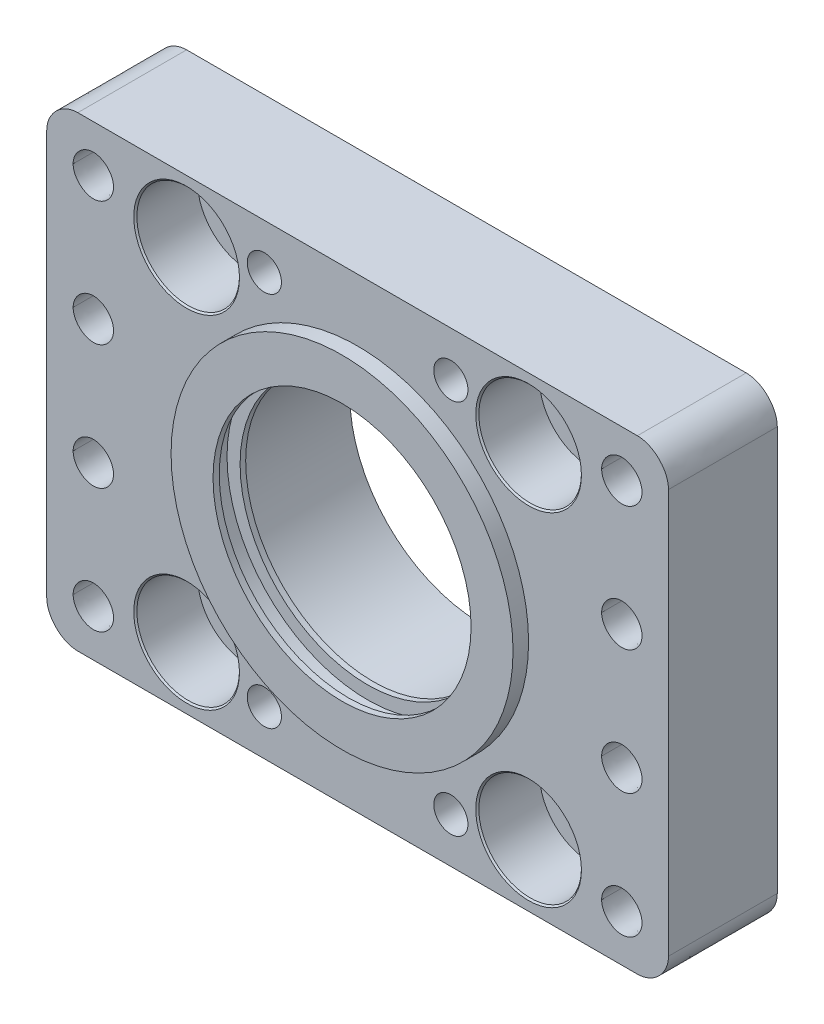
SolidWorks part; units mm, degrees
ref_plane "Front Plane" through (0, 0, 0) normal (0, 0, 1) x (1, 0, 0)
ref_plane "Top Plane" through (0, 0, 0) normal (0, 1, 0) x (1, 0, 0)
ref_plane "Right Plane" through (0, 0, 0) normal (1, 0, 0) x (0, 0, -1)
sketch "Sketch2" plane through (0, 0, 0) normal (0, 0, 1) x (1, 0, 0)
  circle A1 centre (48.7494, 55) radius 8.25
  spline S40 degree 3 poles (-53.0006, -55) (-53.0006, -59.3307) (-56.9229, -63.2494) (-65.5784, -63.2506) (-69.5006, -59.3366) (-69.5006, -55) knots 0 0 0 0 0.5 0.5 1 1 1 1
  spline S41 degree 3 poles (-69.5006, -55) (-69.5006, -50.6693) (-65.5784, -46.7506) (-56.9229, -46.7494) (-53.0006, -50.6634) (-53.0006, -55) knots 0 0 0 0 0.5 0.5 1 1 1 1
  spline S42 degree 3 poles (56.9994, -55) (56.9994, -59.3307) (53.0771, -63.2494) (44.4216, -63.2506) (40.4994, -59.3366) (40.4994, -55) knots 0 0 0 0 0.5 0.5 1 1 1 1
  spline S43 degree 3 poles (40.4994, -55) (40.4994, -50.6693) (44.4216, -46.7506) (53.0771, -46.7494) (56.9994, -50.6634) (56.9994, -55) knots 0 0 0 0 0.5 0.5 1 1 1 1
  spline S46 degree 3 poles (-53.0006, 55) (-53.0006, 50.6693) (-56.9229, 46.7506) (-65.5784, 46.7494) (-69.5006, 50.6634) (-69.5006, 55) knots 0 0 0 0 0.5 0.5 1 1 1 1
  spline S47 degree 3 poles (-69.5006, 55) (-69.5006, 59.3307) (-65.5784, 63.2494) (-56.9229, 63.2506) (-53.0006, 59.3366) (-53.0006, 55) knots 0 0 0 0 0.5 0.5 1 1 1 1
  spline S48 degree 3 poles (-84.7506, -60) (-84.7506, -63.4114) (-87.8428, -66.4994) (-94.6585, -66.5006) (-97.7506, -63.4173) (-97.7506, -60) knots 0 0 0 0 0.5 0.5 1 1 1 1
  spline S49 degree 3 poles (-97.7506, -60) (-97.7506, -56.5886) (-94.6585, -53.5006) (-87.8428, -53.4994) (-84.7506, -56.5827) (-84.7506, -60) knots 0 0 0 0 0.5 0.5 1 1 1 1
  spline S50 degree 3 poles (-84.7506, -20) (-84.7506, -23.4114) (-87.8428, -26.4994) (-94.6585, -26.5006) (-97.7506, -23.4173) (-97.7506, -20) knots 0 0 0 0 0.5 0.5 1 1 1 1
  spline S51 degree 3 poles (-97.7506, -20) (-97.7506, -16.5886) (-94.6585, -13.5006) (-87.8428, -13.4994) (-84.7506, -16.5827) (-84.7506, -20) knots 0 0 0 0 0.5 0.5 1 1 1 1
  spline S52 degree 3 poles (-84.7506, 20) (-84.7506, 16.5886) (-87.8428, 13.5006) (-94.6585, 13.4994) (-97.7506, 16.5827) (-97.7506, 20) knots 0 0 0 0 0.5 0.5 1 1 1 1
  spline S53 degree 3 poles (-97.7506, 20) (-97.7506, 23.4114) (-94.6585, 26.4994) (-87.8428, 26.5006) (-84.7506, 23.4173) (-84.7506, 20) knots 0 0 0 0 0.5 0.5 1 1 1 1
  spline S54 degree 3 poles (-84.7506, 60) (-84.7506, 56.5886) (-87.8428, 53.5006) (-94.6585, 53.4994) (-97.7506, 56.5827) (-97.7506, 60) knots 0 0 0 0 0.5 0.5 1 1 1 1
  spline S55 degree 3 poles (-97.7506, 60) (-97.7506, 63.4114) (-94.6585, 66.4994) (-87.8428, 66.5006) (-84.7506, 63.4173) (-84.7506, 60) knots 0 0 0 0 0.5 0.5 1 1 1 1
  spline S56 degree 3 poles (85.2494, -60) (85.2494, -63.4114) (82.1572, -66.4994) (75.3415, -66.5006) (72.2494, -63.4173) (72.2494, -60) knots 0 0 0 0 0.5 0.5 1 1 1 1
  spline S57 degree 3 poles (72.2494, -60) (72.2494, -56.5886) (75.3415, -53.5006) (82.1572, -53.4994) (85.2494, -56.5827) (85.2494, -60) knots 0 0 0 0 0.5 0.5 1 1 1 1
  spline S58 degree 3 poles (85.2494, -20) (85.2494, -23.4114) (82.1572, -26.4994) (75.3415, -26.5006) (72.2494, -23.4173) (72.2494, -20) knots 0 0 0 0 0.5 0.5 1 1 1 1
  spline S59 degree 3 poles (72.2494, -20) (72.2494, -16.5886) (75.3415, -13.5006) (82.1572, -13.4994) (85.2494, -16.5827) (85.2494, -20) knots 0 0 0 0 0.5 0.5 1 1 1 1
  spline S60 degree 3 poles (85.2494, 20) (85.2494, 16.5886) (82.1572, 13.5006) (75.3415, 13.4994) (72.2494, 16.5827) (72.2494, 20) knots 0 0 0 0 0.5 0.5 1 1 1 1
  spline S61 degree 3 poles (72.2494, 20) (72.2494, 23.4114) (75.3415, 26.4994) (82.1572, 26.5006) (85.2494, 23.4173) (85.2494, 20) knots 0 0 0 0 0.5 0.5 1 1 1 1
  spline S62 degree 3 poles (85.2494, 60) (85.2494, 56.5886) (82.1572, 53.5006) (75.3415, 53.4994) (72.2494, 56.5827) (72.2494, 60) knots 0 0 0 0 0.5 0.5 1 1 1 1
  spline S63 degree 3 poles (72.2494, 60) (72.2494, 63.4114) (75.3415, 66.4994) (82.1572, 66.5006) (85.2494, 63.4173) (85.2494, 60) knots 0 0 0 0 0.5 0.5 1 1 1 1
  spline S72 degree 3 poles (-106.2506, -65) (-106.2506, -21.6667) (-106.2506, 21.6667) (-106.2506, 65) knots 0 0 0 0 1 1 1 1
  spline S73 degree 3 poles (-96.2506, -75) (-101.4866, -75) (-106.2506, -70.236) (-106.2506, -65) knots 0 0 0 0 1 1 1 1
  spline S74 degree 3 poles (-96.2506, -75) (-36.2506, -75) (23.7494, -75) (83.7494, -75) knots 0 0 0 0 1 1 1 1
  spline S75 degree 3 poles (93.7494, -65) (93.7494, -70.236) (88.9853, -75) (83.7494, -75) knots 0 0 0 0 1 1 1 1
  spline S76 degree 3 poles (93.7494, 65) (93.7494, 21.6667) (93.7494, -21.6667) (93.7494, -65) knots 0 0 0 0 1 1 1 1
  spline S77 degree 3 poles (83.7494, 75) (88.9853, 75) (93.7494, 70.236) (93.7494, 65) knots 0 0 0 0 1 1 1 1
  spline S78 degree 3 poles (83.7494, 75) (23.7494, 75) (-36.2506, 75) (-96.2506, 75) knots 0 0 0 0 1 1 1 1
  spline S79 degree 3 poles (-106.2506, 65) (-106.2506, 70.236) (-101.4866, 75) (-96.2506, 75) knots 0 0 0 0 1 1 1 1
  point P43 (0, 0.001)
  point P44 (0.001, 0.001)
  point P45 (0.001, 0)
extrude "Boss-Extrude1" add sketch "Sketch2" along normal blind 35
sketch "Sketch4" plane through (0, 0, 35) normal (0, 0, 1) x (1, 0, 0)
  line L0 (-106.2506, 65) -> (-106.2506, -65) construction
  line L1 (23.7494, 60.5) -> (-36.2506, 60.5) construction
  line L2 (23.7494, 60.5) -> (23.7494, -60.5) construction
  line L3 (23.7494, -60.5) -> (-36.2506, -60.5) construction
  line L4 (-36.2506, 60.5) -> (-36.2506, -60.5) construction
  line L5 (23.7494, 60.5) -> (-36.2506, -60.5) construction
  line L6 (23.7494, -60.5) -> (-36.2506, 60.5) construction
  line L7 (83.7494, 75) -> (-96.2506, 75) construction
  circle A0 centre (-36.2506, 60.5) radius 3.3
  circle A1 centre (23.7494, 60.5) radius 3.3
  circle A2 centre (23.7494, -60.5) radius 3.3
  circle A3 centre (-36.2506, -60.5) radius 3.3
  point P0 (-6.2506, 0)
  dimension "D4" = 6.6
  dimension "D1" = 100
  dimension "D2" = 60
  dimension "D3" = 121
  dimension "D5" = 75
extrude "Cut-Extrude1" cut sketch "Sketch4" against normal blind 35
sketch "Sketch5" plane through (0, 0, 35) normal (0, 0, 1) x (1, 0, 0)
  line L1 (48.7494, -55) -> (-61.2506, -55) construction
  line L2 (48.7494, -55) -> (48.7494, 55) construction
  line L3 (48.7494, 55) -> (-61.2506, 55) construction
  line L4 (-61.2506, -55) -> (-61.2506, 55) construction
  line L5 (48.7494, -55) -> (-61.2506, 55) construction
  line L6 (48.7494, 55) -> (-61.2506, -55) construction
  line L7 (-106.2506, 65) -> (-106.2506, -65) construction
  circle A0 centre (-61.2506, 55) radius 16.5
  circle A1 centre (48.7494, 55) radius 16.5
  circle A2 centre (48.7494, -55) radius 16.5
  circle A3 centre (-61.2506, -55) radius 16.5
  point P0 (-6.2506, 0)
  dimension "D4" = 33
  dimension "D1" = 110
  dimension "D2" = 110
  dimension "D3" = 100
extrude "Cut-Extrude2" cut sketch "Sketch5" against normal blind 20
sketch "Sketch6" plane through (0, 0, 35) normal (0, 0, 1) x (1, 0, 0)
  line L0 (-106.2506, 65) -> (-106.2506, -65) construction
  line L1 (23.7494, 60.5) -> (-36.2506, 60.5) construction
  line L2 (23.7494, 60.5) -> (23.7494, -60.5) construction
  line L3 (23.7494, -60.5) -> (-36.2506, -60.5) construction
  line L4 (-36.2506, 60.5) -> (-36.2506, -60.5) construction
  line L5 (23.7494, 60.5) -> (-36.2506, -60.5) construction
  line L6 (23.7494, -60.5) -> (-36.2506, 60.5) construction
  circle A0 centre (-36.2506, 60.5) radius 5.5
  circle A1 centre (23.7494, 60.5) radius 5.5
  circle A2 centre (23.7494, -60.5) radius 5.5
  circle A3 centre (-36.2506, -60.5) radius 5.5
  point P0 (-6.2506, 0)
  dimension "D4" = 11
  dimension "D5" = 11
  dimension "D1" = 60
  dimension "D2" = 121
  dimension "D3" = 100
extrude "Cut-Extrude3" cut sketch "Sketch6" against normal blind 10
sketch "Sketch7" plane through (0, 0, 0) normal (0, 0, -1) x (-1, 0, 0)
  line L0 (106.2506, -65) -> (106.2506, 65) construction
  circle A1 centre (6.2506, 0) radius 62.5
  dimension "D1" = 125
  dimension "D3" = 100
extrude "Boss-Extrude2" add sketch "Sketch7" along normal blind 5
ref_plane "Plane2" through (0, 0, 17.5) normal (0, 0, 1) x (1, 0, 0)
sketch "Sketch8" plane through (0, 0, 0) normal (0, 0, -1) x (-1, 0, 0)
  line L4 (106.2506, -65) -> (106.2506, 65)
  line L5 (106.2506, -65) -> (106.2506, 65)
  line L6 (96.2506, 75) -> (-83.7494, 75)
  line L7 (96.2506, 75) -> (-83.7494, 75)
  line L8 (-93.7494, 65) -> (-93.7494, -65)
  line L9 (-93.7494, 65) -> (-93.7494, -65)
  line L10 (-83.7494, -75) -> (96.2506, -75)
  line L11 (-83.7494, -75) -> (96.2506, -75)
  spline S4 degree 3 poles (524.8944, 828.4689) (-559.5561, -894.3167) (925.5651, 590.8034) (-797.209, -493.6378) knots -5.020717 -5.020717 -5.020717 -5.020717 6.020697 6.020697 6.020697 6.020697 only from (96.2506, -75) to (106.2506, -65)
  spline S5 degree 3 poles (96.2506, -75) (101.4866, -75) (106.2506, -70.236) (106.2506, -65) knots 0 0 0 0 1 1 1 1
  spline S6 degree 3 poles (-797.2183, 493.6437) (925.5673, -590.8068) (-559.5527, 894.3144) (524.8885, -828.4596) knots -5.020717 -5.020717 -5.020717 -5.020717 6.020697 6.020697 6.020697 6.020697 only from (106.2506, 65) to (96.2506, 75)
  spline S7 degree 3 poles (106.2506, 65) (106.2506, 70.236) (101.4866, 75) (96.2506, 75) knots 0 0 0 0 1 1 1 1
  spline S8 degree 3 poles (-512.3931, -828.4689) (572.0574, 894.3167) (-913.0638, -590.8034) (809.7102, 493.6378) knots -5.020717 -5.020717 -5.020717 -5.020717 6.020697 6.020697 6.020697 6.020697 only from (-83.7494, 75) to (-93.7494, 65)
  spline S9 degree 3 poles (-83.7494, 75) (-88.9853, 75) (-93.7494, 70.236) (-93.7494, 65) knots 0 0 0 0 1 1 1 1
  spline S10 degree 3 poles (809.7196, -493.6437) (-913.066, 590.8068) (572.054, -894.3144) (-512.3872, 828.4596) knots -5.020717 -5.020717 -5.020717 -5.020717 6.020697 6.020697 6.020697 6.020697 only from (-93.7494, -65) to (-83.7494, -75)
  spline S11 degree 3 poles (-93.7494, -65) (-93.7494, -70.236) (-88.9853, -75) (-83.7494, -75) knots 0 0 0 0 1 1 1 1
  dimension "D1" = 0
chamfer "Chamfer2" distance 0.5 angle 45 4 edges at (-44.7506, -55, 35) (-44.7506, 55, 35) (65.2494, -55, 35) (65.2494, 55, 35)
sketch "Sketch9" plane through (0, 0, 35) normal (0, 0, 1) x (1, 0, 0)
  circle A3 centre (-6.2506, 0) radius 55
  dimension "D1" = 110
extrude "Boss-Extrude3" add sketch "Sketch9" along normal blind 5
sketch "Sketch12" plane through (0, 0, -5) normal (0, 0, -1) x (-1, 0, 0)
  circle A0 centre (6.2506, 0) radius 42.5
  dimension "D1" = 85
extrude "Cut-Extrude7" cut sketch "Sketch12" against normal blind 35
sketch "Sketch13" plane through (0, 0, 30) normal (0, 0, -1) x (-1, 0, 0)
  circle A0 centre (6.2506, 0) radius 41
  dimension "D1" = 82
extrude "Cut-Extrude8" cut sketch "Sketch13" against normal blind 35
ref_plane "Plane6" through (0, 0, 31.8) normal (0, 0, -1) x (-1, 0, 0)
sketch "Sketch14" plane through (0, 0, 31.8) normal (0, 0, -1) x (-1, 0, 0)
  circle A0 centre (6.2506, 0) radius 45.2
  dimension "D1" = 90.4
extrude "Cut-Extrude9" cut sketch "Sketch14" against normal blind 6.2
sketch "Sketch15" plane through (0, 0, 38) normal (0, 0, -1) x (-1, 0, 0)
  circle A0 centre (6.2506, 0) radius 41.5
  dimension "D1" = 83
extrude "Cut-Extrude10" cut sketch "Sketch15" against normal blind 6.2
